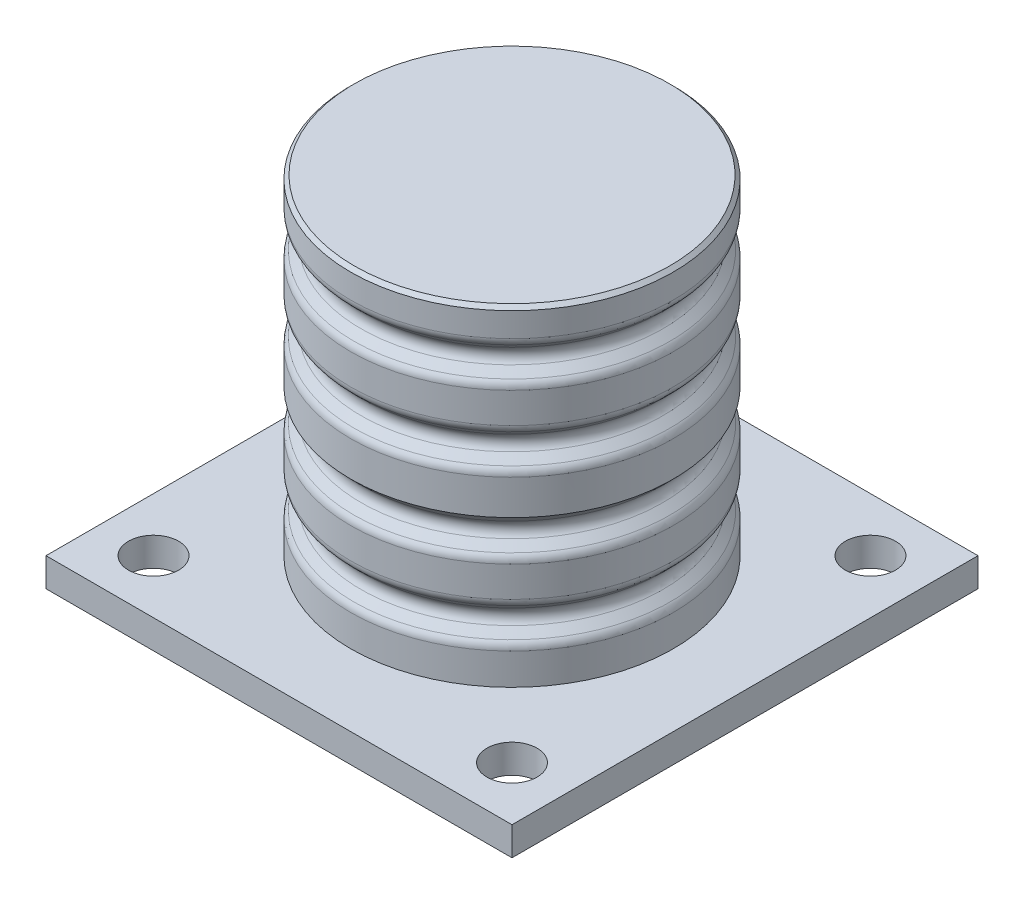
SolidWorks part; units mm, degrees
material "Q235B"
ref_plane "Front Plane" through (0, 0, 0) normal (0, 0, 1) x (1, 0, 0)
ref_plane "Top Plane" through (0, 0, 0) normal (0, 1, 0) x (1, 0, 0)
ref_plane "Right Plane" through (0, 0, 0) normal (1, 0, 0) x (0, 0, -1)
sketch "Sketch2" plane through (0, 0, 0) normal (0, 1, 0) x (1, 0, 0)
  line L1 (65, -65) -> (-65, -65)
  line L2 (65, -65) -> (65, 65)
  line L3 (65, 65) -> (-65, 65)
  line L4 (-65, -65) -> (-65, 65)
  line L5 (65, -65) -> (-65, 65) construction
  line L6 (65, 65) -> (-65, -65) construction
  circle A0 centre (-50, -50) radius 7
  circle A1 centre (-50, 50) radius 7
  circle A2 centre (50, 50) radius 7
  circle A3 centre (50, -50) radius 7
  point P0 (0, 0)
  point P17 (0, 0)
  dimension "D3" = 14
  dimension "D1" = 130
  dimension "D2" = 130
  dimension "D5" = 100
  dimension "D4" = 4
extrude "Boss-Extrude1" add sketch "Sketch2" along normal blind 8
sketch "Sketch3" plane through (0, 0, 0) normal (0, 1, 0) x (1, 0, 0)
  circle A0 centre (0, 0) radius 45
  dimension "D1" = 90
extrude "Boss-Extrude2" add sketch "Sketch3" along normal blind 100
chamfer "Chamfer1" distance 1 angle 45 1 edges at (0, 100, 45)
sketch "Sketch4" plane through (0, 0, 0) normal (0, 0, 1) x (1, 0, 0)
  line L0 (45, 18) -> (40, 23)
  line L1 (45, 8) -> (45, 99) construction
  line L2 (40, 23) -> (45, 28)
  line L3 (-65, 8) -> (65, 8) construction
  line L4 (45, 28) -> (45, 18)
  line L5 (0, 0) -> (0, 48.6715) construction
  line L6 (45, 39) -> (40, 44)
  line L7 (40, 44) -> (45, 49)
  line L8 (45, 49) -> (45, 39)
  line L9 (45, 60) -> (40, 65)
  line L10 (40, 65) -> (45, 70)
  line L11 (45, 70) -> (45, 60)
  line L12 (45, 81) -> (40, 86)
  line L13 (40, 86) -> (45, 91)
  line L14 (45, 91) -> (45, 81)
  line L15 (45, 18) -> (45, 39) construction
  line L16 (45, 23) -> (40, 23) construction
  dimension "D1" = 10
  dimension "D2" = 4
  dimension "D3" = 21
  dimension "D4" = 11
revolve "Cut-Revolve1" cut sketch "Sketch4" angle 360 about L5
fillet "Fillet1" radius 3 11 edges at (0, 18, -45) (0, 28, -45) (0, 39, -45) (0, 60, -45) (0, 70, -45) (0, 81, -45) (0, 91, -45) (0, 86, -40) (0, 65, -40) (0, 23, -40) (0, 44, -40)
